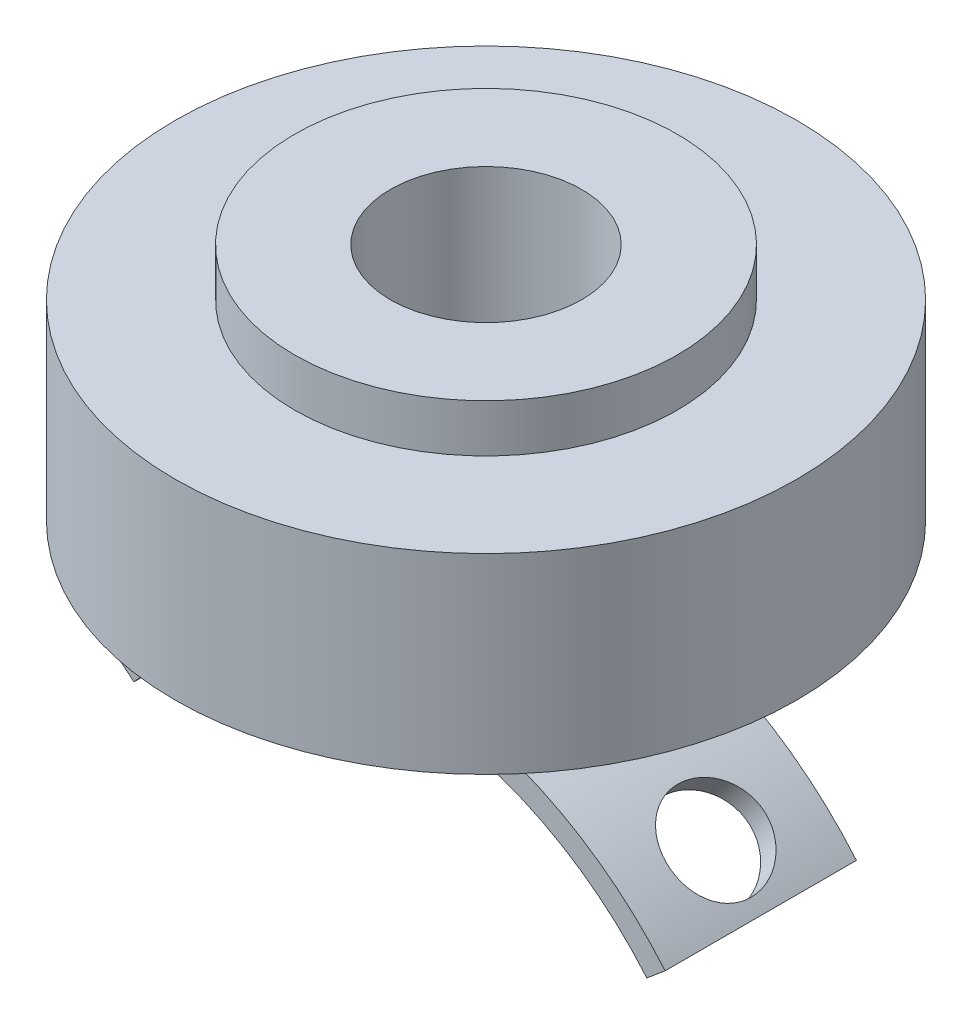
from build123d import *

# Parameters (mm, degrees)
BOSS_EXTRUDE4_DEPTH      = 20
BOSS_EXTRUDE5_REACH      = 41.361
BOSS_EXTRUDE5_END_RADIUS = 37.5
SKETCH8_R                = 10
SKETCH9_R                = 20
BOSS_EXTRUDE6_DEPTH      = 5
SKETCH10_R               = 32.5
BOSS_EXTRUDE7_DEPTH      = 20
SKETCH11_R               = 20
BOSS_EXTRUDE8_DEPTH      = 5
SKETCH12_R               = 10
CUT_EXTRUDE3_DEPTH       = 20


with BuildPart() as part:
    # Sketch4 → Boss-Extrude4 (new body)
    with BuildSketch(Plane.XY):
        with BuildLine():
            Line((-26.811555509, 22.497566339), (-28.726666617, 24.104535363))
            ThreePointArc((-28.726666617, 24.104535363), (0, 37.5), (28.726666617, 24.104535363))
            Line((28.726666617, 24.104535363), (26.811555509, 22.497566339))
            ThreePointArc((26.811555509, 22.497566339), (0, 35), (-26.811555509, 22.497566339))
        make_face()
    extrude(amount=BOSS_EXTRUDE4_DEPTH)

    # Boss-Extrude5: up to this cylinder (the profile starts outside it)
    boss_extrude5_end = Plane(origin=(0, 0, 10), z_dir=(0, 0, -1)) * Cylinder(BOSS_EXTRUDE5_END_RADIUS, 158.722, mode=Mode.PRIVATE)
    # Sketch8 → Boss-Extrude5 (add, up to the surface)
    with BuildSketch(Plane(origin=(0, 40.5, 0), x_dir=(1, 0, 0), z_dir=(0, 1, 0)), mode=Mode.PRIVATE) as boss_extrude5_sk1:
        with Locations(Location((0, -10, 0), (0, 0, 270))):
            Circle(SKETCH8_R)
    boss_extrude5_tool1 = extrude(boss_extrude5_sk1.sketch, amount=-BOSS_EXTRUDE5_REACH, mode=Mode.PRIVATE) - boss_extrude5_end
    add(boss_extrude5_tool1.solids().sort_by_distance((0, 40.5, 10))[0])

    # Sketch9 → Boss-Extrude6 (add)
    with BuildSketch(Plane(origin=(0, 40.5, 0), x_dir=(1, 0, 0), z_dir=(0, 1, 0))):
        with Locations(Location((0, -10, 0), (0, 0, 270))):
            Circle(SKETCH9_R)
    extrude(amount=BOSS_EXTRUDE6_DEPTH)

    # Sketch10 → Boss-Extrude7 (add)
    with BuildSketch(Plane(origin=(0, 45.5, 0), x_dir=(1, 0, 0), z_dir=(0, 1, 0))):
        with Locations(Location((0, -10, 0), (0, 0, 270))):
            Circle(SKETCH10_R)
    extrude(amount=BOSS_EXTRUDE7_DEPTH)

    # Sketch11 → Boss-Extrude8 (add)
    with BuildSketch(Plane(origin=(0, 65.5, 0), x_dir=(1, 0, 0), z_dir=(0, 1, 0))):
        with Locations(Location((0, -10, 0), (0, 0, 270))):
            Circle(SKETCH11_R)
    extrude(amount=BOSS_EXTRUDE8_DEPTH)

    # Sketch12 → Cut-Extrude3 (cut)
    with BuildSketch(Plane(origin=(0, 70.5, 0), x_dir=(1, 0, 0), z_dir=(0, 1, 0))):
        with Locations(Location((0, -10, 0), (0, 0, 270))):
            Circle(SKETCH12_R)
    extrude(amount=-CUT_EXTRUDE3_DEPTH, mode=Mode.SUBTRACT)

    # Sketch15 → Cut-Revolve3 (revolve, cut)
    with BuildSketch(Plane.XY.offset(10), mode=Mode.PRIVATE) as cut_revolve3_sk:
        Polygon((-17.693131792, 21.085853377), (-26.278152948, 31.317083182), (-30.108375164, 28.103145134), (-21.523354007, 17.871915328), align=None)
    revolve(cut_revolve3_sk.sketch.rotate(Axis((-17.693131792, 21.085853377, 10), (-0.6427876096865413, 0.7660444431189765, 0)), 180), axis=Axis((-17.693131792, 21.085853377, 10), (-0.6427876096865413, 0.7660444431189765, 0)), mode=Mode.SUBTRACT)

    # Sketch16 → Cut-Revolve4 (revolve, cut)
    with BuildSketch(Plane.XY.offset(10), mode=Mode.PRIVATE) as cut_revolve4_sk:
        Polygon((17.792638641, 21.204441023), (27.637153268, 32.936676696), (23.806931052, 36.150614744), (13.962416426, 24.418379071), align=None)
    revolve(cut_revolve4_sk.sketch.rotate(Axis((17.792638641, 21.204441023, 10), (0.6427876096865399, 0.7660444431189776, 0)), 180), axis=Axis((17.792638641, 21.204441023, 10), (0.6427876096865399, 0.7660444431189776, 0)), mode=Mode.SUBTRACT)


solid = part.part
